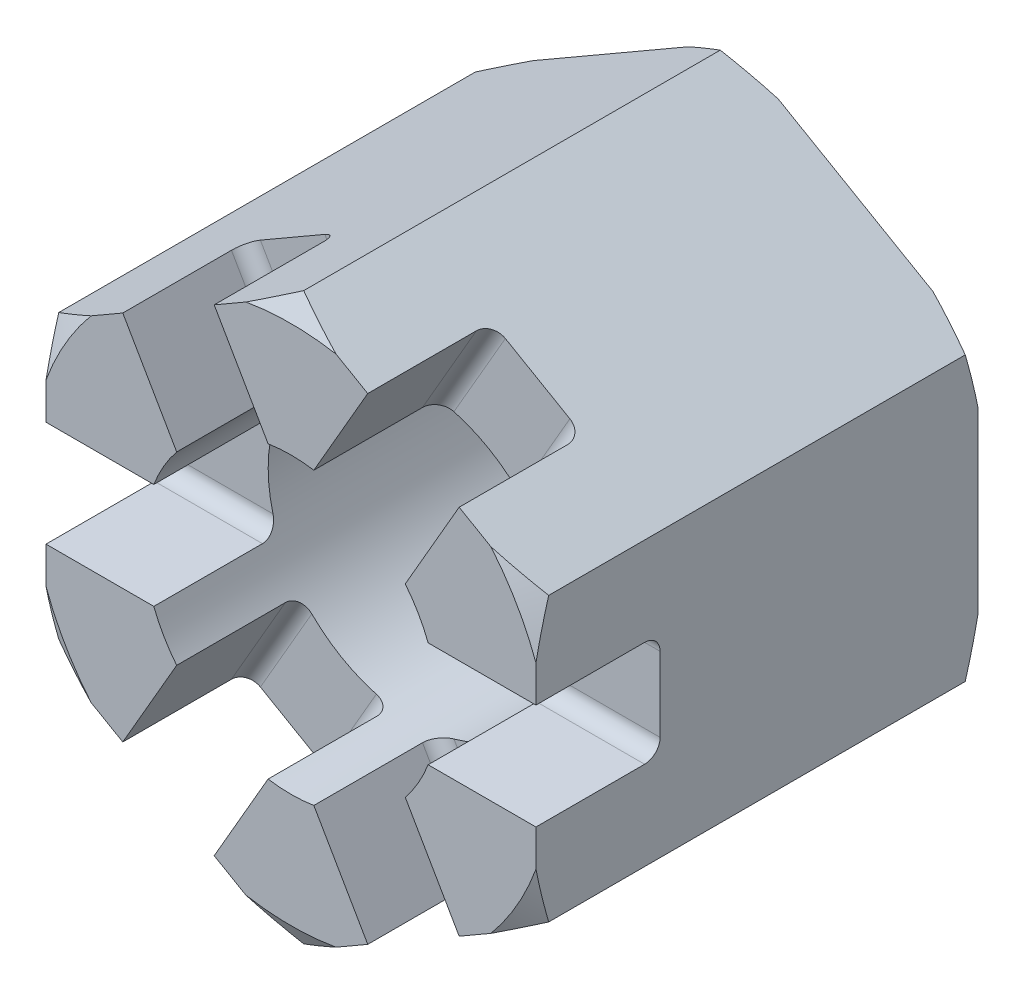
SolidWorks part; units mm, degrees
material "Q235"
ref_plane "Plane1" through (0, 0, 0) normal (0, 0, 1) x (1, 0, 0)
ref_plane "Plane2" through (0, 0, 0) normal (0, 1, 0) x (1, 0, 0)
ref_plane "Plane3" through (0, 0, 0) normal (1, 0, 0) x (0, 0, -1)
sketch "Dimension sketch" plane through (0, 0, 0) normal (0, 0, 1) x (1, 0, 0)
  line L0 (0, 0) -> (21, 0) construction
  line L1 (22.78, 0) -> (37.88, 0) construction
  line L2 (37.88, 0) -> (57.08, 0) construction
  line L3 (-11.3333, 0) -> (2, 0) construction
  line L4 (0, 0) -> (22.78, 0) construction
  line L5 (-11.3333, 0) -> (-11.3333, 9.7) construction
  point P3 (14, 0)
  point P4 (2, 0)
  point P5 (22.78, 0)
  point P6 (17.8, 0)
  point P8 (21, 0)
  point P15 (35.58, 0)
  point P16 (42.13, 0)
  dimension "D1" = 13.3333
  dimension "D" = 14
  dimension "P" = 2
  dimension "e(min)" = 22.78
  dimension "m(max)" = 17.8
  dimension "s(max)" = 21
  dimension "da(max)" = 15.1
  dimension "dw(min)" = 19.2
  dimension "w(max)" = 12.8
  dimension "n(max)" = 4.25
  dimension "m´(min)" = 9.7
sketch "Sketch1" plane through (0, 0, 0) normal (0, 0, 1) x (1, 0, 0)
  line L0 (-9.864, 0) -> (9.864, 0) construction
  line L1 (0, 11.39) -> (0, -11.39) construction
  line L3 (0, 11.39) -> (-9.864, 5.695)
  line L4 (-9.864, 5.695) -> (-9.864, -5.695)
  line L5 (-9.864, -5.695) -> (0, -11.39)
  line L6 (0, -11.39) -> (9.864, -5.695)
  line L7 (9.864, -5.695) -> (9.864, 5.695)
  line L8 (9.864, 5.695) -> (0, 11.39)
  circle A0 centre (0, 0) radius 9.864 construction
  circle A1 centre (0, 0) radius 5.9175
  dimension "D" = 11.835
  dimension "e" = 22.78
extrude "Base-Extrude" add sketch "Sketch1" along normal blind 17.8
cosmetic thread "Cosmetic Thread1" parameters "D2"=14
sketch "Sketch2" plane through (0, 0, 0) normal (0, 0, -1) x (-1, 0, 0)
  circle A0 centre (0, 0) radius 10.5
  circle A1 centre (0, 0) radius 5.9175 construction
  dimension "s" = 21
extrude "Cut-Extrude1" cut sketch "Sketch2" against normal through all draft 60 flip side to cut
sketch "Sketch3" plane through (0, 0, 17.8) normal (0, 0, 1) x (1, 0, 0)
  circle A0 centre (0, 0) radius 10.5
  dimension "D1" = 21
extrude "Cut-Extrude2" cut sketch "Sketch3" against normal through all draft 60 flip side to cut
sketch "Sketch6" plane through (9.864, 0, 0) normal (1, 0, 0) x (0, 0, -1)
  line L0 (-14.9451, 0) -> (3.4921, 0) construction
  line L1 (-17.8, 0) -> (0, 0) construction
  line L3 (-17.8, -3.5987) -> (-17.8, 3.5987) construction
  line L4 (-17.8, -2.125) -> (-17.8, 2.125)
  line L5 (-17.8, 2.125) -> (-13.425, 2.125)
  line L6 (-12.8, -1.5) -> (-12.8, 1.5)
  line L7 (0, -3.5987) -> (0, 3.5987) construction
  line L8 (-17.8, -2.125) -> (-13.425, -2.125)
  arc A0 (-13.425, 2.125) -> (-12.8, 1.5) centre (-13.425, 1.5) cw
  arc A1 (-13.425, -2.125) -> (-12.8, -1.5) centre (-13.425, -1.5) ccw
  point P14 (-12.8, 2.125)
  point P17 (-12.8, -2.125)
  dimension "D1" = 0.625
  dimension "W" = 12.8
  dimension "n" = 2.125
extrude "Cut-Extrude3" cut sketch "Sketch6" against normal through all
pattern_circular "CirPattern1" count 3 over 360 about axis through (0, 0, 0) along (0, 0, 1) of "Cut-Extrude3"
chamfer "Chamfer1" distance 0.2208 angle 45 1 edges at (5.9175, 0, 0)
